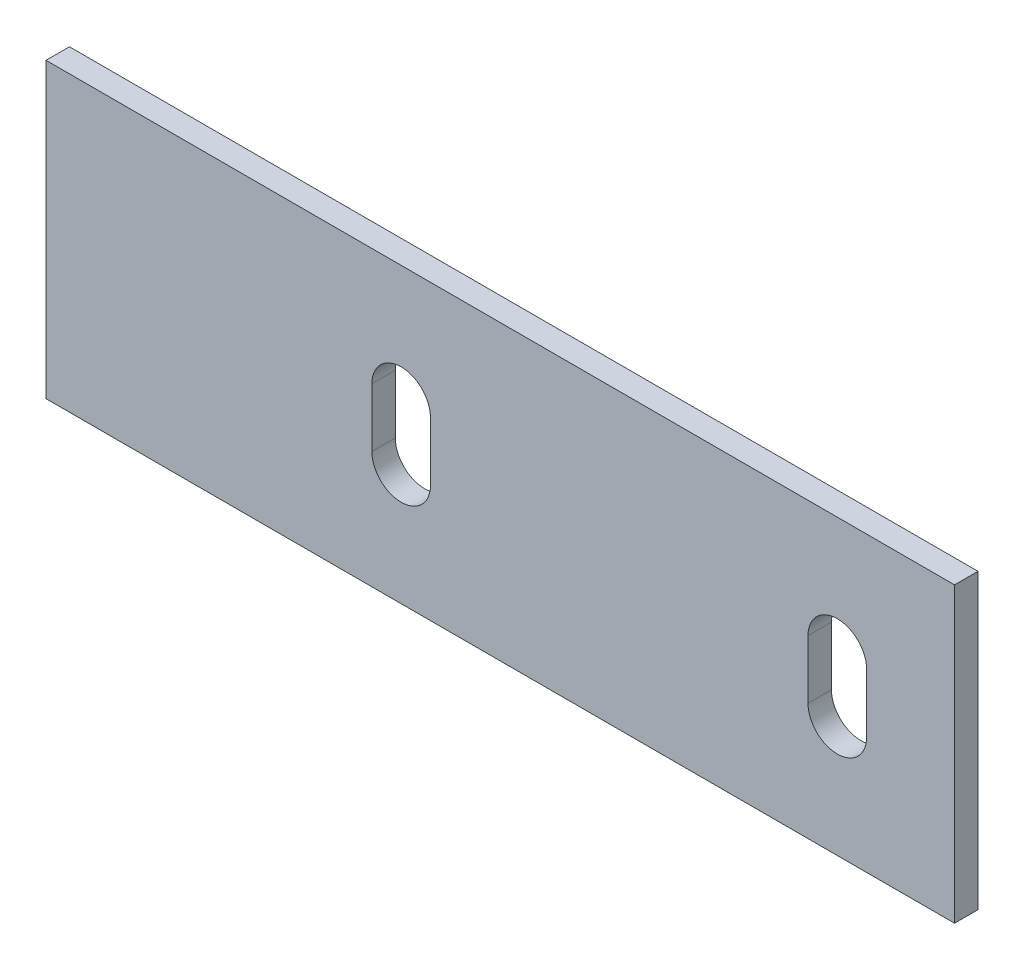
from build123d import *

# Parameters (mm, degrees)
BOSS_EXTRUDE1_DEPTH = 20


with BuildPart() as part:
    # Sketch1 → Boss-Extrude1 (new body)
    with BuildSketch(Plane.XY):
        Polygon((14040.331499194, 4658.160293083), (14040.331499194, 4408.160293083), (13265.233105958, 4408.160293083), (13265.233105872, 4658.160293083), align=None)
        with BuildLine():
            Line((13543.233105077, 4558.160293388), (13543.233105077, 4508.160293551))
            ThreePointArc((13543.233105077, 4508.160293551), (13568.233205921, 4483.160293631), (13593.233104917, 4508.160495399))
            Line((13593.233104917, 4508.160495399), (13593.233104917, 4558.159705819))
            ThreePointArc((13593.233104917, 4558.159705819), (13568.233398781, 4583.159999523), (13543.233105077, 4558.160293388))
        make_face(mode=Mode.SUBTRACT)
        with BuildLine():
            Line((13915.331499495, 4558.160293394), (13915.331499495, 4508.160293549))
            ThreePointArc((13915.331499495, 4508.160293549), (13940.331591876, 4483.160293859), (13965.331499344, 4508.160478461))
            Line((13965.331499344, 4508.160478461), (13965.331499344, 4558.159730803))
            ThreePointArc((13965.331499344, 4558.159730803), (13940.331780715, 4583.160012023), (13915.331499495, 4558.160293394))
        make_face(mode=Mode.SUBTRACT)
    extrude(amount=BOSS_EXTRUDE1_DEPTH)


solid = part.part
